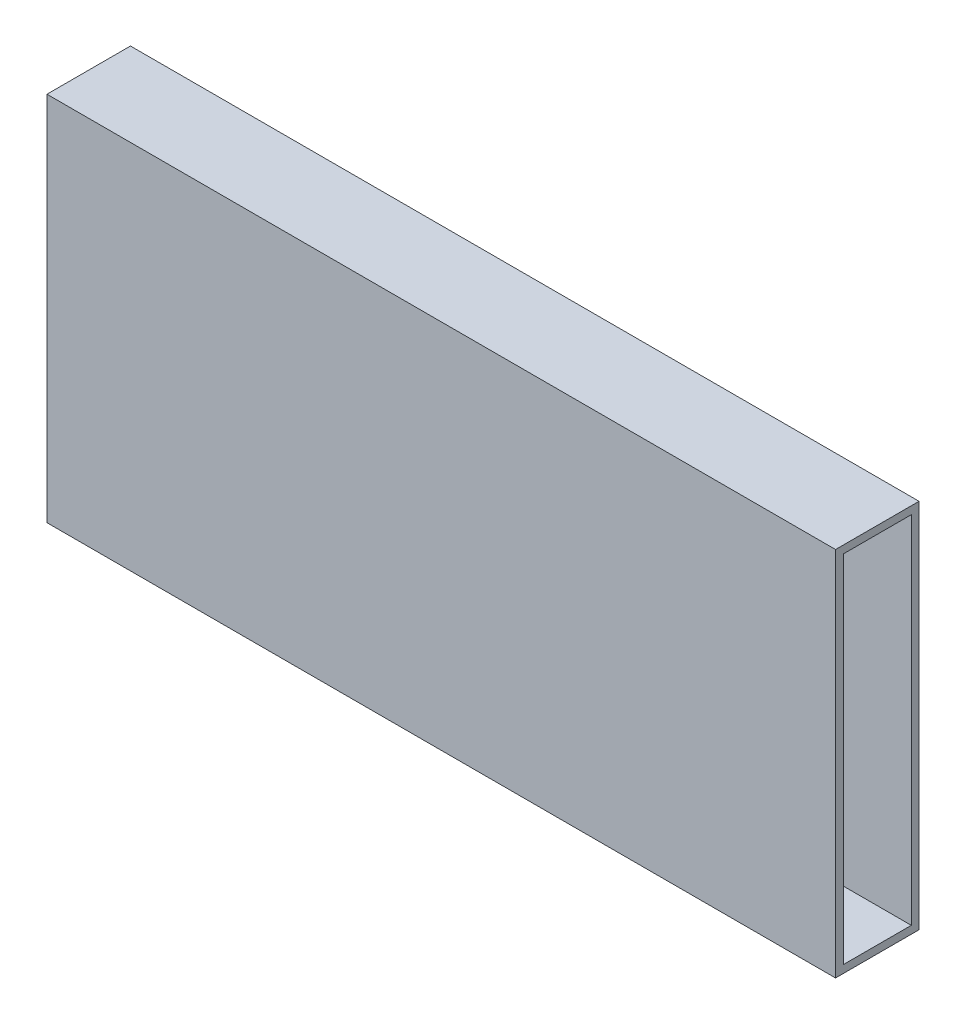
from build123d import *

# Parameters (mm, degrees)
SKETCH1_W           = 1020
SKETCH1_H           = 480
BOSS_EXTRUDE1_DEPTH = 108
SHELL1_T            = -10
SKETCH2_R           = 18.75
CUT_EXTRUDE1_DEPTH  = 10


with BuildPart() as part:
    # Sketch1 → Boss-Extrude1 (new body)
    with BuildSketch(Plane.XY):
        Rectangle(SKETCH1_W, SKETCH1_H)
    extrude(amount=BOSS_EXTRUDE1_DEPTH)

    # Shell1
    shell1_openings = [part.faces().sort_by_distance(p)[0] for p in [
        (-510, 0, 54),
        (510, 0, 54),
    ]]
    offset(amount=SHELL1_T, openings=shell1_openings, kind=Kind.INTERSECTION)

    # Sketch2 → Cut-Extrude1 (cut)
    with BuildSketch(Plane(origin=(0, 0, 0), x_dir=(-1, 0, 0), z_dir=(0, 0, -1))):
        with Locations((-397.470896816, 192.1875)):
            Circle(SKETCH2_R)
        with Locations((-395.533103518, -192.1875)):
            Circle(SKETCH2_R)
        with Locations((465.091896482, -191.83711567)):
            Circle(SKETCH2_R)
        with Locations((465.091896482, 191.83711567)):
            Circle(SKETCH2_R)
    extrude(amount=-CUT_EXTRUDE1_DEPTH, mode=Mode.SUBTRACT)


solid = part.part
